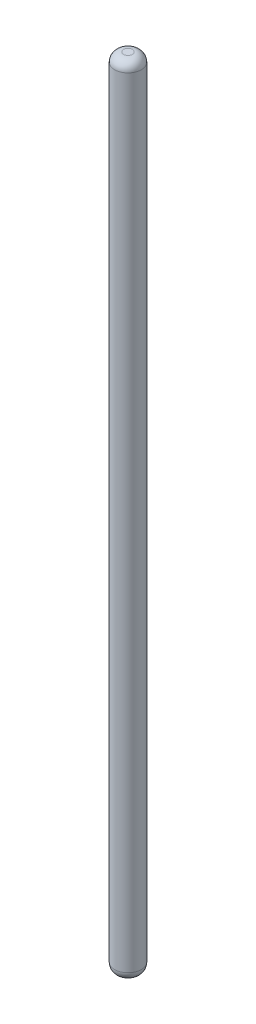
from build123d import *

# Parameters (mm, degrees)
SKETCH1_R           = 3
BOSS_EXTRUDE1_DEPTH = 180
FILLET1_R           = 2


with BuildPart() as part:
    # Sketch1 → Boss-Extrude1 (new body)
    with BuildSketch(Plane(origin=(0, 0, 0), x_dir=(1, 0, 0), z_dir=(0, 1, 0))):
        with Locations(Location((0, 0, 0), (0, 0, 90))):
            Circle(SKETCH1_R)
    extrude(amount=BOSS_EXTRUDE1_DEPTH)

    # Fillet1
    fillet1_edges = [part.edges().sort_by_distance(p)[0] for p in [
        (0, 0, 3),
        (0, 180, 3),
    ]]
    fillet(fillet1_edges, radius=FILLET1_R)


solid = part.part
